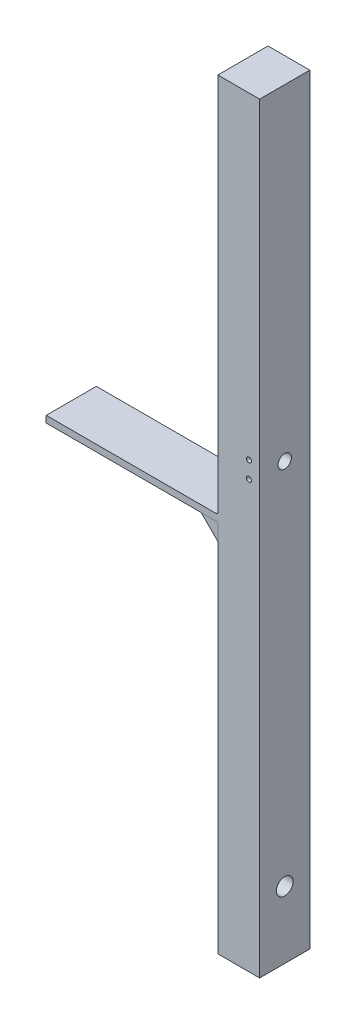
SolidWorks part; units mm, degrees
material "AISI 1045 钢，冷拔"
ref_plane "前视基准面" through (0, 0, 0) normal (0, 0, 1) x (1, 0, 0)
ref_plane "上视基准面" through (0, 0, 0) normal (0, 1, 0) x (1, 0, 0)
ref_plane "右视基准面" through (0, 0, 0) normal (1, 0, 0) x (0, 0, -1)
other "Configuration Table"
sketch "草图1" plane through (0, 0, 0) normal (0, 0, 1) x (1, 0, 0)
  line L0 (0, 0) -> (0, 246.0326)
  line L1 (0, 246.0326) -> (25, 246.0326)
  line L2 (25, 246.0326) -> (25, -38.9674)
  line L5 (25, -53.9674) -> (0, -53.9674)
  line L6 (0, -53.9674) -> (0, 0)
  line L7 (25, -38.9674) -> (25, -53.9674)
  dimension "D1" = 25
  dimension "D4" = 300
extrude "凸台-拉伸2" add sketch "草图1" along normal mid plane 30
sketch "草图2" plane through (0, 0, 0) normal (-1, 0, 0) x (0, 0, 1)
  line L0 (15, -53.9674) -> (-15, -53.9674) construction
  circle A0 centre (0, -13.9674) radius 5
  circle A1 centre (0, 206.0326) radius 4
  dimension "D2" = 10
  dimension "D3" = 8
  dimension "D1" = 40
  dimension "D4" = 220
extrude "切除-拉伸1" cut sketch "草图2" against normal mid plane 132
sketch "草图3" plane through (0, 0, -15) normal (0, 0, -1) x (-1, 0, 0)
  line L0 (0, 173.5326) -> (102.6, 173.5326)
  line L1 (0, 246.0326) -> (0, -53.9674) construction
  line L2 (102.6, 173.5326) -> (102.6, 169.5326)
  line L3 (102.6, 169.5326) -> (0, 169.5326)
  line L4 (102.6, 173.5326) -> (8.6, 173.5326) construction
  line L5 (0, 173.5326) -> (0, 169.5326)
  line L6 (102.6, 178.5326) -> (102.6, 173.5326) construction
  dimension "D1" = 4
extrude "凸台-拉伸3" add sketch "草图3" against normal up to surface (30 mm away) up to face at (12.5, 96.0326, 15)
sketch "草图4" plane through (0, 246.0326, 0) normal (0, 1, 0) x (1, 0, 0)
  line L4 (25, 15) -> (0, 15)
  line L5 (0, 15) -> (0, -15)
  line L6 (0, -15) -> (25, -15)
  line L7 (25, -15) -> (25, 15)
  line L8 (25, 15) -> (0, 15)
  line L9 (0, 15) -> (0, -15)
  line L10 (0, -15) -> (25, -15)
  line L11 (25, -15) -> (25, 15)
  dimension "D1" = 0
extrude "凸台-拉伸4" add sketch "草图4" along normal blind 155
sketch "草图5" plane through (0, 0, -15) normal (0, 0, -1) x (-1, 0, 0)
  circle A0 centre (-18.6, 201.0326) radius 1
  circle A1 centre (-18.6, 211.0326) radius 1
  dimension "D1" = 2
  dimension "D2" = 2
extrude "切除-拉伸2" cut sketch "草图5" against normal blind 10
sketch "草图6" plane through (0, 0, 15) normal (0, 0, 1) x (1, 0, 0)
  circle A0 centre (18.6, 201.0326) radius 1.5
  circle A1 centre (18.6, 211.0326) radius 1.5
  dimension "D1" = 3
  dimension "D2" = 3
extrude "切除-拉伸3" cut sketch "草图6" against normal blind 10
other "角撑板1" parameters "D1"=5, "D2"=5, "D3"=0, "D4"=0, "D10"=5, "D11"=10, "D12"=10, "D13"=15, "D14"=45, "D15"=15
sketch "草图7" plane through (0, 169.5326, -15) normal (0, 0, 1) x (1, 0, 0)
  line L0 (0, 0) -> (-10, 0)
  line L1 (0, 0) -> (0, -10)
  line L2 (-10, 0) -> (0, -10)
other "角撑板2" parameters "D1"=5, "D2"=5, "D3"=0, "D4"=0, "D10"=5, "D11"=10, "D12"=10, "D13"=15, "D14"=45, "D15"=15
sketch "草图8" plane through (0, 169.5326, 15) normal (0, 0, -1) x (-1, 0, 0)
  line L0 (0, 0) -> (10, 0)
  line L1 (0, 0) -> (0, -10)
  line L2 (10, 0) -> (0, -10)
fillet "圆角1" radius 1 1 edges at (0, 173.5326, 0)
